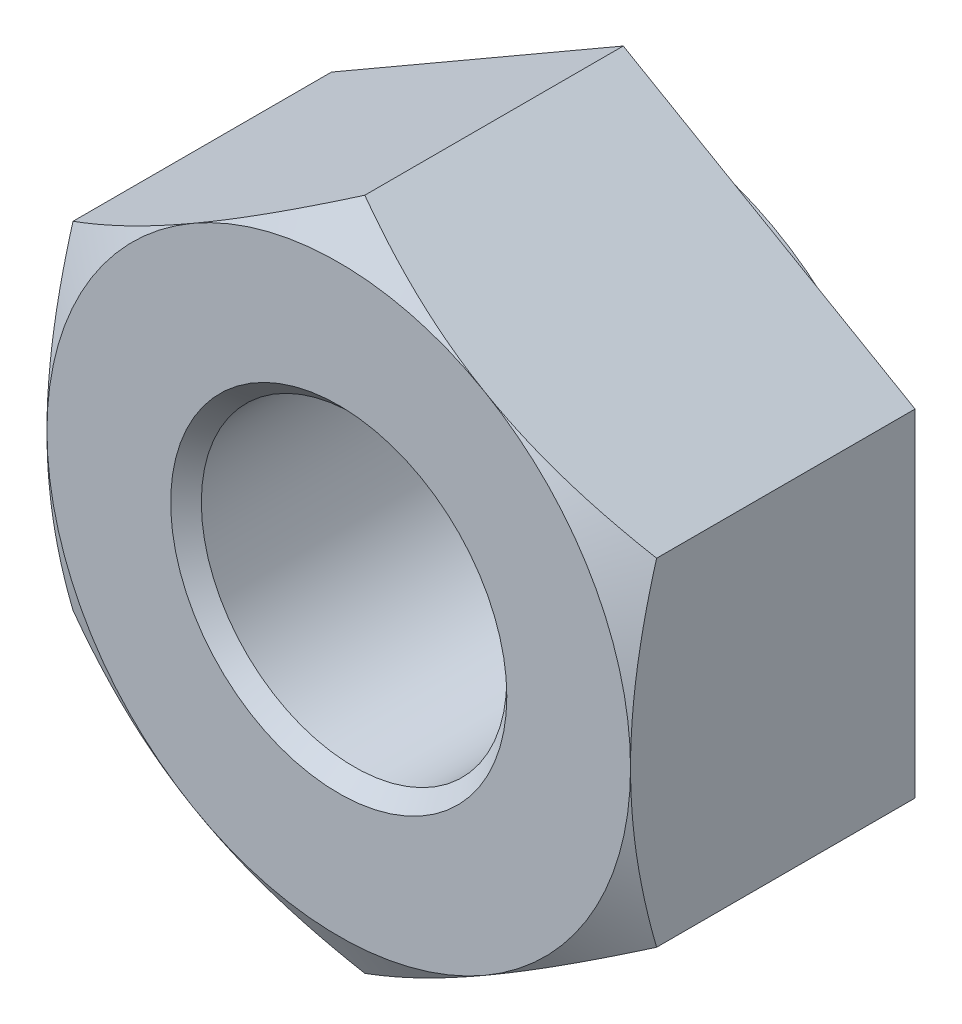
from build123d import *

# Parameters (mm, degrees)
SKETCH1_R          = 4.188125
EXTRUDE1_DEPTH     = 8.4
SKETCH2_OUTSIDE_W  = 23.168
SKETCH2_OUTSIDE_H  = 25.644
SKETCH2_OUTSIDE_R  = 7.3
CUT_EXTRUDE2_DEPTH = 0.6
SKETCH3_OUTSIDE_W  = 78.002
SKETCH3_OUTSIDE_H  = 80.478
SKETCH3_OUTSIDE_R  = 8
CUT_EXTRUDE3_DEPTH = 15.828800806
CUT_EXTRUDE3_DRAFT = -60
CHAMFER1_SIZE      = 0.42


with BuildPart() as part:
    # Sketch1 → Extrude1 (new body)
    with BuildSketch(Plane.XY):
        Polygon((0, 9.237604307), (-8, 4.618802154), (-8, -4.618802154), (0, -9.237604307), (8, -4.618802154), (8, 4.618802154), align=None)
        Circle(SKETCH1_R, mode=Mode.SUBTRACT)
    extrude(amount=EXTRUDE1_DEPTH)

    # Sketch2 outside → Cut-Extrude2 (cut)
    with BuildSketch(Plane.XY):
        Rectangle(SKETCH2_OUTSIDE_W, SKETCH2_OUTSIDE_H)
        Circle(SKETCH2_OUTSIDE_R, mode=Mode.SUBTRACT)
    extrude(amount=CUT_EXTRUDE2_DEPTH, mode=Mode.SUBTRACT)


with BuildPart() as cut_extrude3_tool:
    # Sketch3 outside → Cut-Extrude3 (with draft: the straight prism first)
    with BuildSketch(Plane.XY.offset(8.4)):
        Rectangle(SKETCH3_OUTSIDE_W, SKETCH3_OUTSIDE_H)
        Circle(SKETCH3_OUTSIDE_R, mode=Mode.SUBTRACT)
    extrude(amount=-CUT_EXTRUDE3_DEPTH)
    # Cut-Extrude3: the draft: its side faces are tilted about the plane it starts from
    cut_extrude3_sides = [cut_extrude3_tool.faces().sort_by_distance(p)[0] for p in [
        (0, -40.239, 0.485599597),
        (39.001, 0, 0.485599597),
        (0, 40.239, 0.485599597),
        (-39.001, 0, 0.485599597),
        (-8, 0, 0.485599597),
    ]]
    draft(cut_extrude3_sides, Plane.XY.offset(8.4), CUT_EXTRUDE3_DRAFT)


with BuildPart() as part_1:
    add(part.part)

    # Cut-Extrude3: cut by cut_extrude3_tool
    add(cut_extrude3_tool.part, mode=Mode.SUBTRACT)

    # Chamfer1
    chamfer1_edges = [part_1.edges().sort_by_distance(p)[0] for p in [
        (-4.188125, 0, 0),
        (-4.188125, 0, 8.4),
    ]]
    chamfer(chamfer1_edges, length=CHAMFER1_SIZE)


solid = part_1.part
